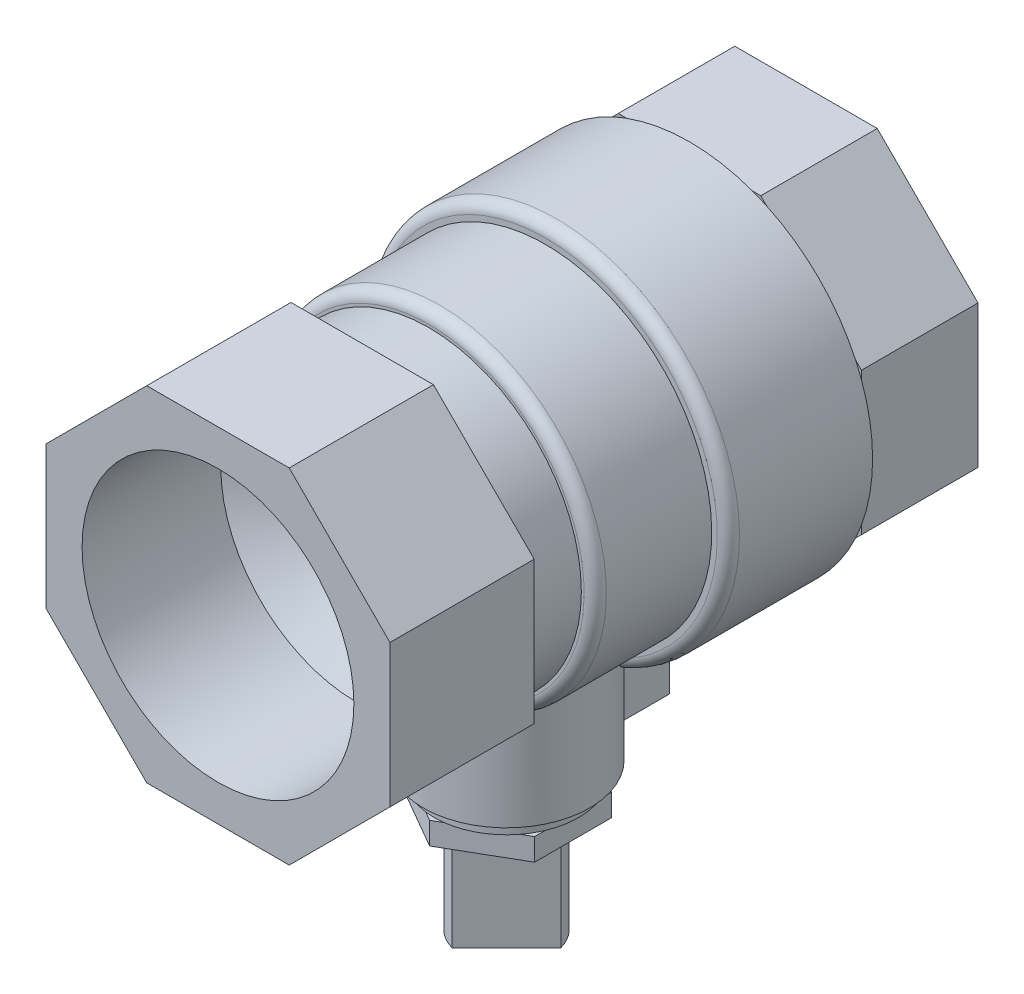
from build123d import *

# Parameters (mm, degrees)
SKETCH_1_R               = 15
EXTRUDE_1_DEPTH          = 10.5
SKETCH_2_R               = 13.75
EXTRUDE_2_DEPTH          = 6
EXTRUDE_3_DEPTH          = 13
SKETCH_4_R               = 16.5
EXTRUDE_4_DEPTH          = 13
EXTRUDE_5_DEPTH          = 10.5
FILLET_1_R               = 1
HOLE_WIZARD_G3_4_1_D     = 24.5
HOLE_WIZARD_G3_4_1_DEPTH = 12.5
HOLE_WIZARD_G3_4_1_TIP   = 7.360542583
HOLE_WIZARD_G3_4_2_D     = 24.5
HOLE_WIZARD_G3_4_2_DEPTH = 12.5
HOLE_WIZARD_G3_4_2_TIP   = 7.360542583
CUT_EXTRUDE_1_REACH      = 59.909
SKETCH_11_R              = 7.5
EXTRUDE_6_REACH          = 54.369
SKETCH_13_R              = 6.5
EXTRUDE_7_DEPTH          = 1.25
EXTRUDE_8_DEPTH          = 2
SKETCH_15_R              = 4
EXTRUDE_9_DEPTH          = 10
CUT_EXTRUDE_START        = -10
CUT_EXTRUDE_2_DEPTH      = 10


with BuildPart() as part:
    # 草图1 → 凸台-拉伸1 (new body)
    with BuildSketch(Plane.XY):
        with Locations(Location((0, 0, 0), (0, 0, 180))):
            Circle(SKETCH_1_R)
    extrude(amount=EXTRUDE_1_DEPTH)

    # 草图2 → 凸台-拉伸2 (add)
    with BuildSketch(Plane.XY.offset(10.5)):
        Circle(SKETCH_2_R)
    extrude(amount=EXTRUDE_2_DEPTH)

    # 草图3 → 凸台-拉伸3 (add)
    with BuildSketch(Plane.XY.offset(16.5)):
        Polygon((6.420310217, -15.5), (15.5, -6.420310217), (15.5, 6.420310217), (6.420310217, 15.5), (-6.420310217, 15.5), (-15.5, 6.420310217), (-15.5, -6.420310217), (-6.420310217, -15.5), align=None)
    extrude(amount=EXTRUDE_3_DEPTH)

    # 草图4 → 凸台-拉伸4 (add)
    with BuildSketch(Plane(origin=(0, 0, 0), x_dir=(-1, 0, 0), z_dir=(0, 0, -1))):
        with Locations(Location((0, 0, 0), (0, 0, 180))):
            Circle(SKETCH_4_R)
    extrude(amount=EXTRUDE_4_DEPTH)

    # 草图6 → 凸台-拉伸5 (add)
    with BuildSketch(Plane(origin=(0, 0, -13), x_dir=(-1, 0, 0), z_dir=(0, 0, -1))):
        Polygon((15.5, -6.420310217), (15.5, 6.420310217), (6.420310217, 15.5), (-6.420310217, 15.5), (-15.5, 6.420310217), (-15.5, -6.420310217), (-6.420310217, -15.5), (6.420310217, -15.5), align=None)
    extrude(amount=EXTRUDE_5_DEPTH)

    # 圆角1
    fillet_1_edges = [part.edges().sort_by_distance(p)[0] for p in [
        (-16.5, 0, 0),
        (15, 0, 10.5),
    ]]
    fillet(fillet_1_edges, radius=FILLET_1_R)

    # G3/4 螺纹孔1
    with Locations(Plane.XY.offset(29.5)):
        with Locations((0, 0)):
            Hole(HOLE_WIZARD_G3_4_1_D / 2, depth=HOLE_WIZARD_G3_4_1_DEPTH)
            with Locations((0, 0, -(HOLE_WIZARD_G3_4_1_DEPTH + HOLE_WIZARD_G3_4_1_TIP / 2))):  # 118° drill point
                Cone(0, HOLE_WIZARD_G3_4_1_D / 2, HOLE_WIZARD_G3_4_1_TIP, mode=Mode.SUBTRACT)

    # G3/4 螺纹孔2
    with Locations(Plane(origin=(0, 0, -23.5), x_dir=(-1, 0, 0), z_dir=(0, 0, -1))):
        with Locations((0, 0)):
            Hole(HOLE_WIZARD_G3_4_2_D / 2, depth=HOLE_WIZARD_G3_4_2_DEPTH)
            with Locations((0, 0, -(HOLE_WIZARD_G3_4_2_DEPTH + HOLE_WIZARD_G3_4_2_TIP / 2))):  # 118° drill point
                Cone(0, HOLE_WIZARD_G3_4_2_D / 2, HOLE_WIZARD_G3_4_2_TIP, mode=Mode.SUBTRACT)

    # 切除-拉伸1: up to this cone (the profile starts outside it)
    cut_extrude_1_end = Plane(origin=(0, 0, -23.5), z_dir=(0, 0, 1)).offset(33.139458417) * Cone(1.664e-06, 45.384140214, 27.269541583, align=(Align.CENTER, Align.CENTER, Align.MIN), mode=Mode.PRIVATE)
    # 草图11 → 切除-拉伸1 (cut, up to the surface)
    with BuildSketch(Plane(origin=(0, 0, -23.5), x_dir=(-1, 0, 0), z_dir=(0, 0, -1)), mode=Mode.PRIVATE) as cut_extrude_1_sk1:
        Circle(SKETCH_11_R)
    cut_extrude_1_tool1 = extrude(cut_extrude_1_sk1.sketch, amount=-CUT_EXTRUDE_1_REACH, mode=Mode.PRIVATE) - cut_extrude_1_end
    add(cut_extrude_1_tool1.solids().sort_by_distance((0, 0, -23.5))[0], mode=Mode.SUBTRACT)

    # 草图12 → 凸台-拉伸6 (add, up to next)
    with BuildSketch(Plane(origin=(0, -23.5, 0), x_dir=(-1, 0, 0), z_dir=(0, -1, 0)), mode=Mode.PRIVATE) as extrude_6_sk1:
        with BuildLine():
            Line((-2.2, 9), (2.2, 9))
            Line((2.2, 9), (2.2, 3.670076708))
            ThreePointArc((2.2, 3.670076708), (0, -11), (-2.2, 3.670076708))
            Line((-2.2, 3.670076708), (-2.2, 9))
        make_face()
    extrude_6_tool1 = extrude(extrude_6_sk1.sketch, amount=-EXTRUDE_6_REACH, mode=Mode.PRIVATE) - part.part
    add(extrude_6_tool1.solids().sort_by_distance((0, -23.5, 2.377731))[0])

    # 草图13 → 凸台-拉伸7 (add)
    with BuildSketch(Plane.XZ.offset(23.5)):
        with Locations((0, 3.5)):
            Circle(SKETCH_13_R)
    extrude(amount=EXTRUDE_7_DEPTH)

    # 草图14 → 凸台-拉伸8 (add)
    with BuildSketch(Plane.XZ.offset(24.75)):
        Polygon((6, 6.964101615), (0, 10.42820323), (-6, 6.964101615), (-6, 0.035898385), (0, -3.42820323), (6, 0.035898385), align=None)
    extrude(amount=EXTRUDE_8_DEPTH)

    # 草图15 → 凸台-拉伸9 (add)
    with BuildSketch(Plane.XZ.offset(26.75)):
        with Locations((0, 3.5)):
            Circle(SKETCH_15_R)
    extrude(amount=EXTRUDE_9_DEPTH)

    # 草图16 → 切除-拉伸2 (cut)
    with BuildSketch(Plane.XZ.offset(36.75).offset(CUT_EXTRUDE_START)):
        with BuildLine():
            Line((-3.863703305, 4.53527618), (1.03527618, -0.363703305))
            ThreePointArc((1.03527618, -0.363703305), (-2.828427125, 0.671572875), (-3.863703305, 4.53527618))
        make_face()
        with BuildLine():
            Line((-1.03527618, 7.363703305), (3.863703305, 2.46472382))
            ThreePointArc((3.863703305, 2.46472382), (2.828427125, 6.328427125), (-1.03527618, 7.363703305))
        make_face()
    extrude(amount=CUT_EXTRUDE_2_DEPTH, mode=Mode.SUBTRACT)


solid = part.part
